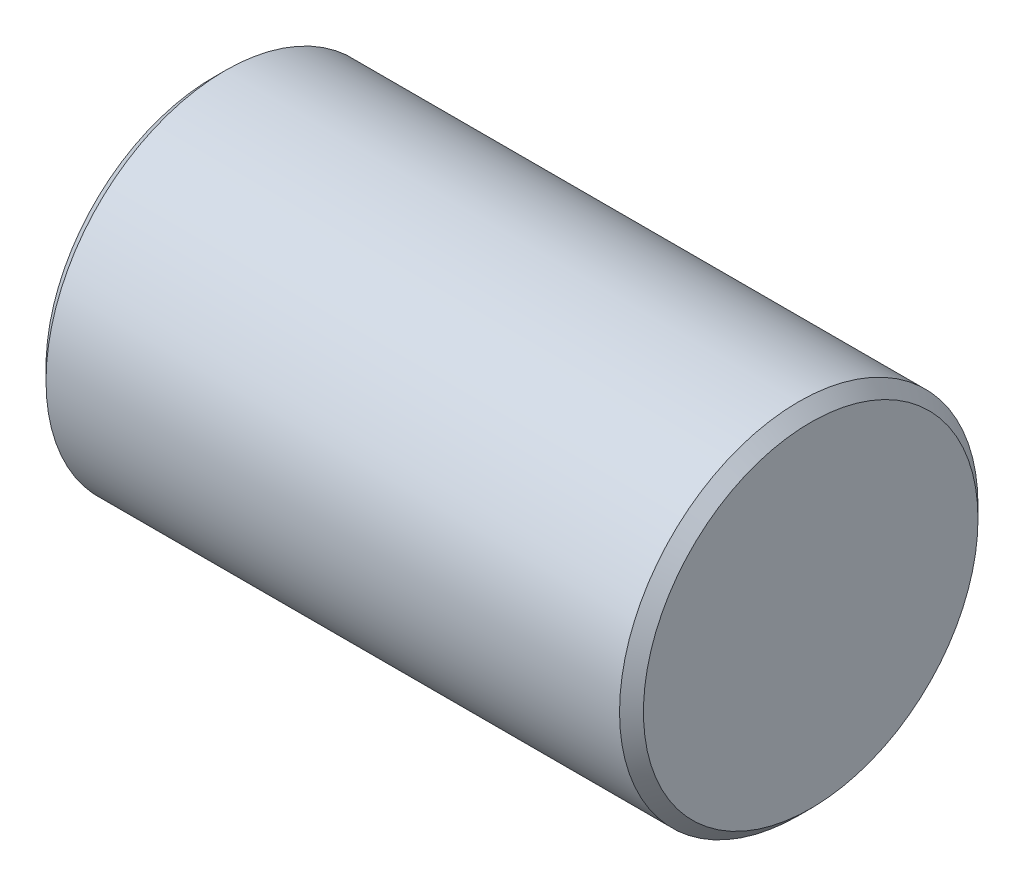
SolidWorks part; units mm, degrees
ref_plane "前视基准面" through (0, 0, 0) normal (0, 0, 1) x (1, 0, 0)
ref_plane "上视基准面" through (0, 0, 0) normal (0, 1, 0) x (1, 0, 0)
ref_plane "右视基准面" through (0, 0, 0) normal (1, 0, 0) x (0, 0, -1)
sketch "草图1" plane through (0, 0, 0) normal (1, 0, 0) x (0, 0, -1)
  circle A0 centre (0, 0) radius 15
extrude "凸台-拉伸1" add sketch "草图1" along normal blind 50
chamfer "倒角1" distance 1 angle 45 2 edges at (0, 0, -15) (50, 0, -15)
